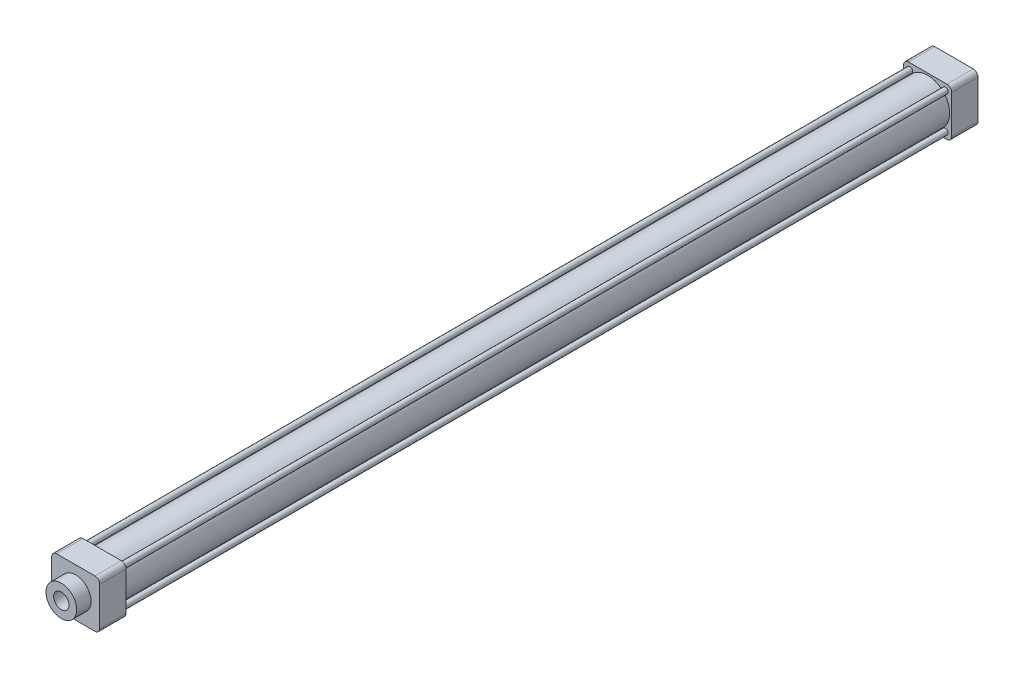
SolidWorks part; units mm, degrees
ref_plane "Front Plane" through (0, 0, 0) normal (0, 0, 1) x (1, 0, 0)
ref_plane "Top Plane" through (0, 0, 0) normal (0, 1, 0) x (1, 0, 0)
ref_plane "Right Plane" through (0, 0, 0) normal (1, 0, 0) x (0, 0, -1)
sketch "Sketch1" plane through (0, 0, 0) normal (0, 0, 1) x (1, 0, 0)
  line L1 (-25, 25) -> (25, 25)
  line L2 (-25, 25) -> (-25, -25)
  line L3 (-25, -25) -> (25, -25)
  line L4 (25, 25) -> (25, -25)
  line L5 (-25, 25) -> (25, -25) construction
  line L6 (-25, -25) -> (25, 25) construction
  point P0 (0, 0)
  dimension "D1" = 50
  dimension "D2" = 50
extrude "Boss-Extrude1" add sketch "Sketch1" along normal blind 27.5
sketch "Sketch2" plane through (0, 0, 27.5) normal (0, 0, 1) x (1, 0, 0)
  circle A0 centre (0, 0) radius 20
  circle A1 centre (0, 0) radius 23
  dimension "D1" = 40
  dimension "D2" = 46
extrude "Boss-Extrude2" add sketch "Sketch2" along normal blind 860
sketch "Sketch3" plane through (0, 0, 887.5) normal (0, 0, 1) x (1, 0, 0)
  line L1 (-25, 25) -> (25, 25)
  line L2 (-25, 25) -> (-25, -25)
  line L3 (-25, -25) -> (25, -25)
  line L4 (25, 25) -> (25, -25)
  line L5 (-25, 25) -> (25, -25) construction
  line L6 (-25, -25) -> (25, 25) construction
  point P0 (0, 0)
  dimension "D1" = 50
  dimension "D2" = 50
extrude "Boss-Extrude3" add sketch "Sketch3" along normal blind 27.5
sketch "Sketch4" plane through (0, 0, 915) normal (0, 0, 1) x (1, 0, 0)
  circle A0 centre (0, 0) radius 16
  dimension "D1" = 32
extrude "Boss-Extrude4" add sketch "Sketch4" along normal blind 15
sketch "Sketch5" plane through (0, 0, 930) normal (0, 0, 1) x (1, 0, 0)
  circle A0 centre (0, 0) radius 8
  dimension "D1" = 16
extrude "Cut-Extrude1" cut sketch "Sketch5" against normal blind 100
sketch "Sketch6" plane through (0, 0, 915) normal (0, 0, 1) x (1, 0, 0)
  circle A0 centre (-18.5, 18.5) radius 3
  circle A1 centre (18.5, 18.5) radius 3
  circle A2 centre (18.5, -18.5) radius 3
  circle A3 centre (-18.5, -18.5) radius 3
  dimension "D1" = 18.5
  dimension "D2" = 18.5
  dimension "D3" = 6
  dimension "D4" = 2
  dimension "D5" = 2
extrude "Boss-Extrude5" add sketch "Sketch6" against normal up to surface (915 mm away) up to face at (0, 0, 0)
fillet "Fillet1" radius 5 8 edges at (-25, -25, 13.75) (-25, -25, 901.25) (25, -25, 13.75) (25, -25, 901.25) (-25, 25, 901.25) (-25, 25, 13.75) (25, 25, 13.75) (25, 25, 901.25)
